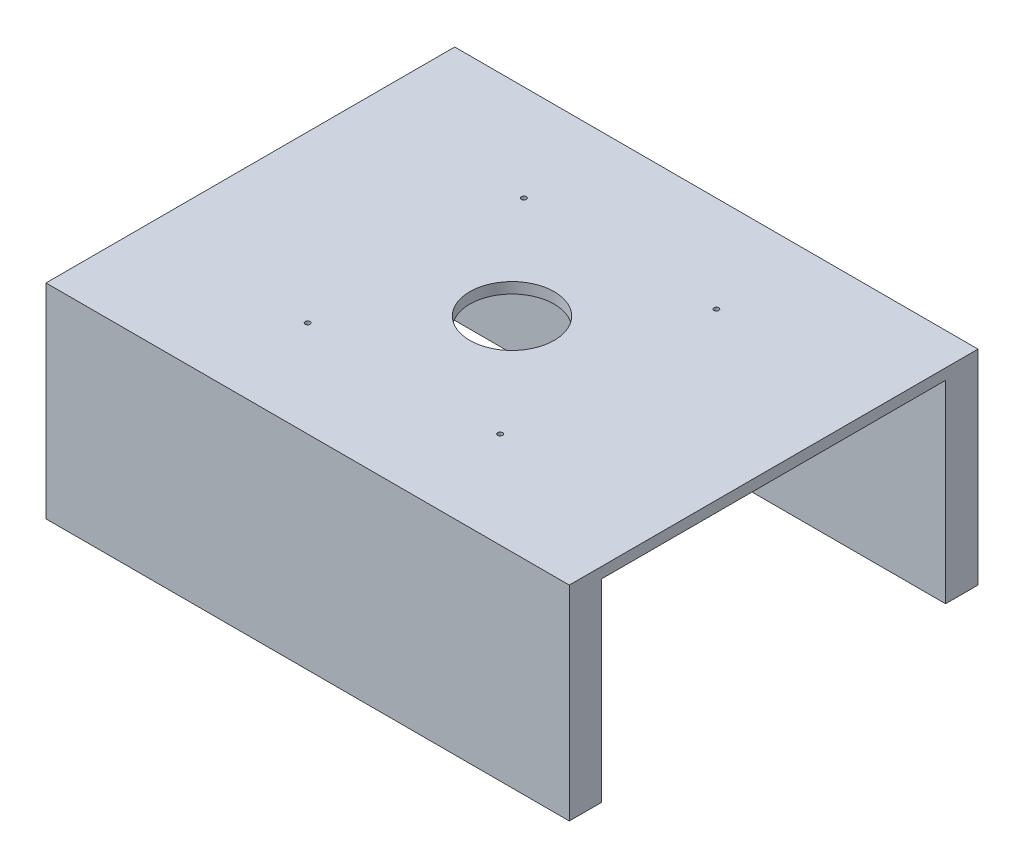
SolidWorks part; units mm, degrees
ref_plane "Front Plane" through (0, 0, 0) normal (0, 0, 1) x (1, 0, 0)
ref_plane "Top Plane" through (0, 0, 0) normal (0, 1, 0) x (1, 0, 0)
ref_plane "Right Plane" through (0, 0, 0) normal (1, 0, 0) x (0, 0, -1)
sketch "Sketch1" plane through (0, 0, 0) normal (0, 1, 0) x (1, 0, 0)
  line L1 (-242, -189) -> (242, -189)
  line L2 (-242, -189) -> (-242, 189)
  line L3 (-242, 189) -> (242, 189)
  line L4 (242, -189) -> (242, 189)
  line L5 (-242, -189) -> (242, 189) construction
  line L6 (-242, 189) -> (242, -189) construction
  point P0 (0, 0)
  dimension "D1" = 378
  dimension "D2" = 484
extrude "Boss-Extrude1" add sketch "Sketch1" along normal blind 189
sketch "Sketch2" plane through (-242, 0, 0) normal (-1, 0, 0) x (0, 0, 1)
  line L0 (-189, 0) -> (189, 0) construction
  line L1 (-159, 0) -> (159, 0)
  line L2 (-159, 0) -> (-159, 179)
  line L3 (-159, 179) -> (159, 179)
  line L4 (159, 0) -> (159, 179)
  line L5 (-189, 189) -> (189, 189) construction
  line L6 (189, 189) -> (189, 0) construction
  line L7 (-189, 189) -> (-189, 0) construction
  dimension "D1" = 10
  dimension "D2" = 30
  dimension "D3" = 30
extrude "Cut-Extrude1" cut sketch "Sketch2" against normal through all
sketch "Sketch3" plane through (0, 189, 0) normal (0, 1, 0) x (1, 0, 0)
  circle A0 centre (-89, -100) radius 2.25
  circle A1 centre (89, -100) radius 2.25
  circle A2 centre (-89, 100) radius 2.25
  circle A3 centre (89, 100) radius 2.25
  circle A4 centre (0, 0) radius 39.0566
  dimension "D1" = 4.5
  dimension "D2" = 178
  dimension "D3" = 178
  dimension "D4" = 89
  dimension "D5" = 89
  dimension "D6" = 200
  dimension "D7" = 200
  dimension "D8" = 100
extrude "Cut-Extrude2" cut sketch "Sketch3" against normal through all
